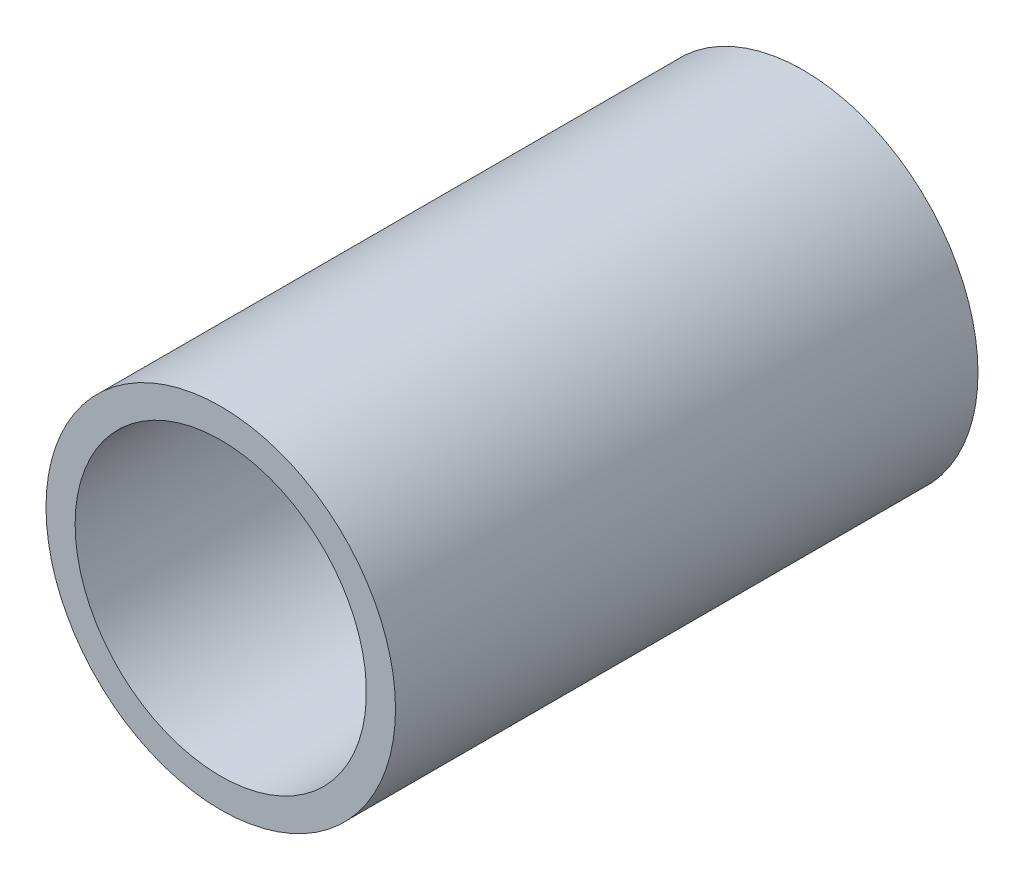
SolidWorks part; units mm, degrees
material "普通碳钢"
ref_plane "Front Plane" through (0, 0, 0) normal (0, 0, 1) x (1, 0, 0)
ref_plane "Top Plane" through (0, 0, 0) normal (0, 1, 0) x (1, 0, 0)
ref_plane "Right Plane" through (0, 0, 0) normal (1, 0, 0) x (0, 0, -1)
sketch "Sketch1" plane through (0, 0, 0) normal (0, 0, 1) x (1, 0, 0)
  circle A0 centre (0, 0) radius 15
  circle A1 centre (0, 0) radius 12.5
  dimension "D1" = 30
  dimension "D2" = 25
extrude "Boss-Extrude1" add sketch "Sketch1" along normal blind 50
